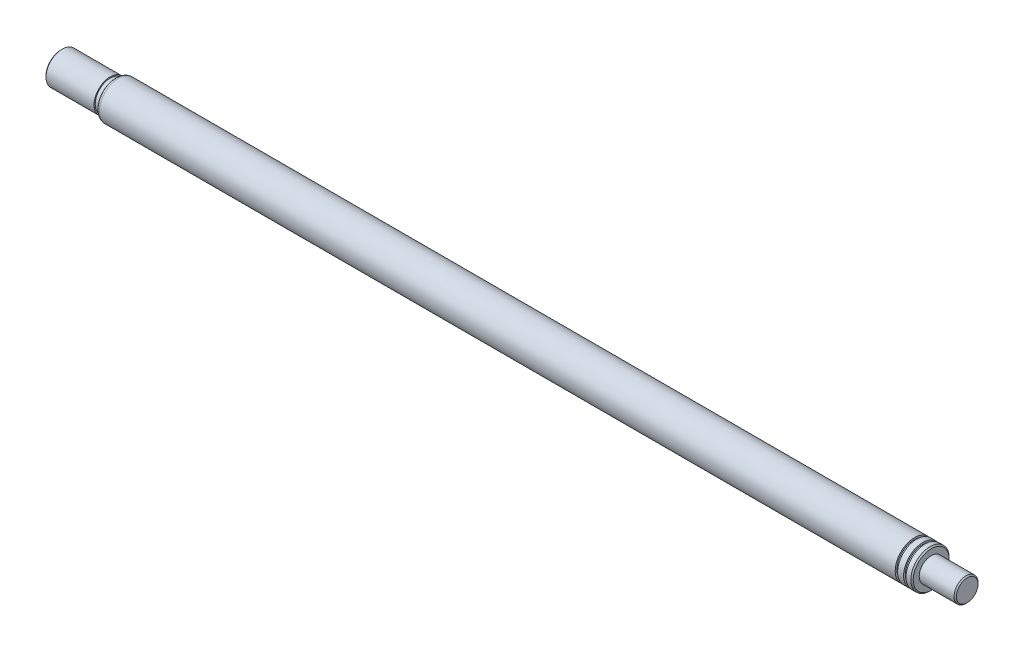
SolidWorks part; units mm, degrees
ref_plane "前视基准面" through (0, 0, 0) normal (0, 0, 1) x (1, 0, 0)
ref_plane "上视基准面" through (0, 0, 0) normal (0, 1, 0) x (1, 0, 0)
ref_plane "右视基准面" through (0, 0, 0) normal (1, 0, 0) x (0, 0, -1)
other "Configuration Table"
sketch "草图1" plane through (0, 0, 0) normal (0, 0, 1) x (1, 0, 0)
  line L0 (0, 0) -> (755, 0) construction
  line L1 (0, 0) -> (0, 12.5)
  line L2 (1, 13.5) -> (41, 13.5)
  line L3 (41, 13.5) -> (41, 12.5)
  line L4 (41, 12.5) -> (45, 12.5)
  line L5 (45, 12.5) -> (45, 13)
  line L6 (48, 16) -> (711, 16)
  line L7 (711, 16) -> (711, 14.5)
  line L8 (711, 14.5) -> (713, 14.5)
  line L9 (713, 14.5) -> (713, 16)
  line L10 (713, 16) -> (718, 16)
  line L11 (718, 16) -> (718, 14.5)
  line L12 (718, 14.5) -> (720, 14.5)
  line L13 (720, 14.5) -> (720, 16)
  line L14 (720, 16) -> (724, 16)
  line L15 (725, 15) -> (725, 10)
  line L16 (725, 10) -> (754, 10)
  line L17 (755, 9) -> (755, 0)
  line L18 (0, 0) -> (755, 0)
  line L19 (0, 12.5) -> (1, 13.5)
  line L20 (724, 16) -> (725, 15)
  line L21 (754, 10) -> (755, 9)
  arc A0 (45, 13) -> (48, 16) centre (48, 13) cw
  point P3 (0, 13.5)
  point P17 (725, 16)
  point P19 (755, 10)
  dimension "D10" = 3
  dimension "D1" = 29
  dimension "D2" = 20
  dimension "D3" = 30
  dimension "D4" = 5
  dimension "D5" = 5
  dimension "D6" = 2
  dimension "D7" = 2
  dimension "D8" = 27
  dimension "D9" = 4
  dimension "D11" = 1
  dimension "D12" = 755
  dimension "D13" = 680
  dimension "D14" = 32
  dimension "D15" = 0.5
revolve "旋转1" add sketch "草图1" angle 360 about L0
